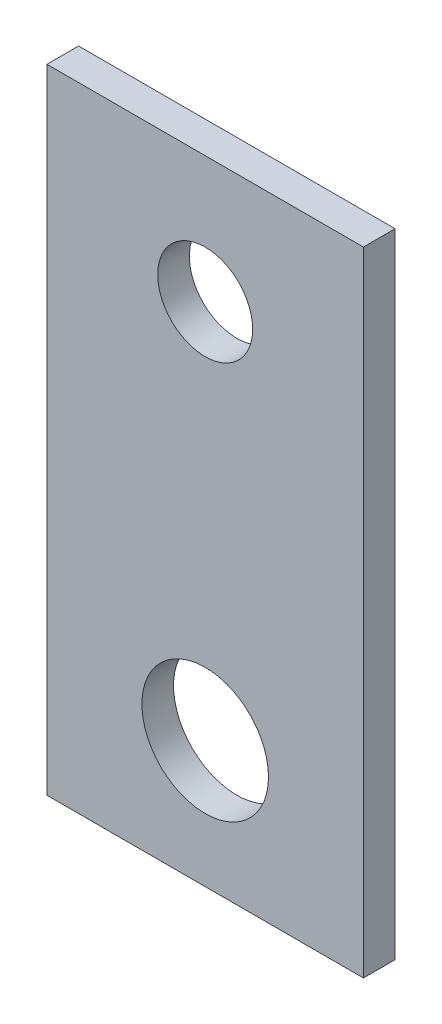
SolidWorks part; units mm, degrees
ref_plane "Front Plane" through (0, 0, 0) normal (0, 0, 1) x (1, 0, 0)
ref_plane "Top Plane" through (0, 0, 0) normal (0, 1, 0) x (1, 0, 0)
ref_plane "Right Plane" through (0, 0, 0) normal (1, 0, 0) x (0, 0, -1)
sketch "Sketch1" plane through (0, 0, 0) normal (0, 0, 1) x (1, 0, 0)
  line L1 (25, 50) -> (-25, 50)
  line L2 (25, 50) -> (25, -50)
  line L3 (25, -50) -> (-25, -50)
  line L4 (-25, 50) -> (-25, -50)
  line L5 (25, 50) -> (-25, -50) construction
  line L6 (25, -50) -> (-25, 50) construction
  point P0 (0, 0)
  dimension "D1" = 50
  dimension "D2" = 100
extrude "Boss-Extrude1" add sketch "Sketch1" along normal blind 5
sketch "Sketch2" plane through (0, 0, 5) normal (0, 0, 1) x (1, 0, 0)
  circle A1 centre (0, -30) radius 10
  circle A2 centre (0, 30) radius 7.5
  dimension "D1" = 15
  dimension "D2" = 20
  dimension "D3" = 60
  dimension "D4" = 30
extrude "Cut-Extrude1" cut sketch "Sketch2" against normal blind 5
